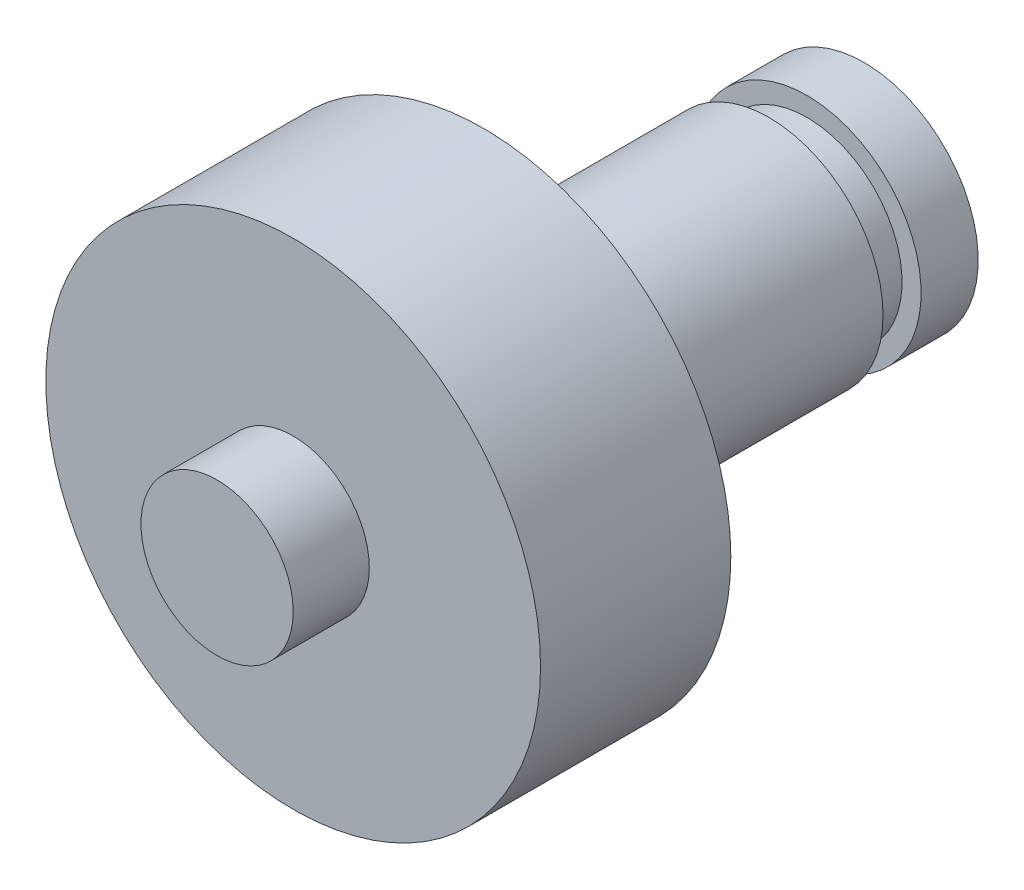
SolidWorks part; units mm, degrees
ref_plane "Front Plane" through (0, 0, 0) normal (0, 0, 1) x (1, 0, 0)
ref_plane "Top Plane" through (0, 0, 0) normal (0, 1, 0) x (1, 0, 0)
ref_plane "Right Plane" through (0, 0, 0) normal (1, 0, 0) x (0, 0, -1)
sketch "Sketch1" plane through (0, 0, 0) normal (0, 0, 1) x (1, 0, 0)
  circle A0 centre (0, 0) radius 6.5
  dimension "D1" = 13
extrude "Extrude1" add sketch "Sketch1" along normal blind 5
sketch "Sketch2" plane through (0, 0, 5) normal (0, 0, 1) x (1, 0, 0)
  circle A0 centre (0, 0) radius 2
  dimension "D1" = 4
extrude "Extrude2" add sketch "Sketch2" along normal blind 2
sketch "Sketch3" plane through (0, 0, 0) normal (0, 0, -1) x (-1, 0, 0)
  circle A0 centre (0, 0) radius 3
  dimension "D1" = 6
extrude "Extrude3" add sketch "Sketch3" along normal blind 7.5
sketch "Sketch4" plane through (0, 0, -7.5) normal (0, 0, -1) x (-1, 0, 0)
  circle A0 centre (0, 0) radius 2.5
  dimension "D1" = 5
extrude "Extrude5" add sketch "Sketch4" along normal blind 1
sketch "Sketch6" plane through (0, 0, -8.5) normal (0, 0, -1) x (-1, 0, 0)
  circle A0 centre (0, 0) radius 3
  dimension "D1" = 6
extrude "Extrude6" add sketch "Sketch6" along normal blind 1.5
